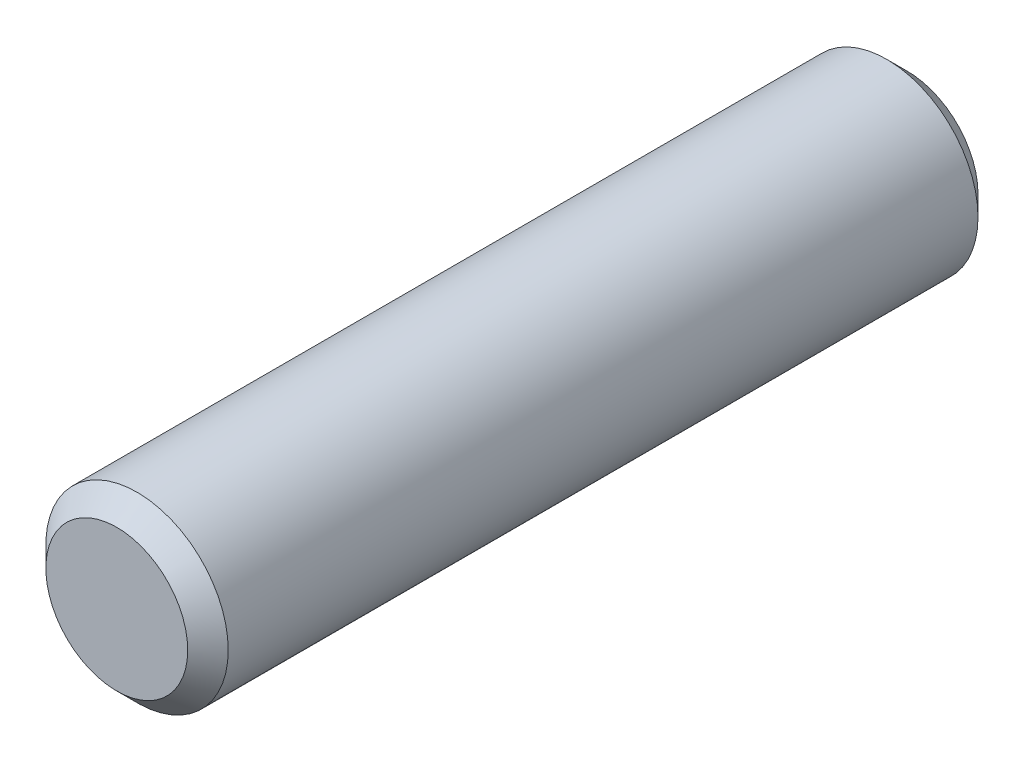
from build123d import *

# Parameters (mm, degrees)
SKETCH1_R           = 4.5
BOSS_EXTRUDE1_DEPTH = 39
CHAMFER1_SIZE       = 1


with BuildPart() as part:
    # Sketch1 → Boss-Extrude1 (new body)
    with BuildSketch(Plane.XY):
        Circle(SKETCH1_R)
    extrude(amount=BOSS_EXTRUDE1_DEPTH)

    # Chamfer1
    chamfer1_edges = [part.edges().sort_by_distance(p)[0] for p in [
        (-4.5, 0, 0),
        (-4.5, 0, 39),
    ]]
    chamfer(chamfer1_edges, length=CHAMFER1_SIZE)


solid = part.part
